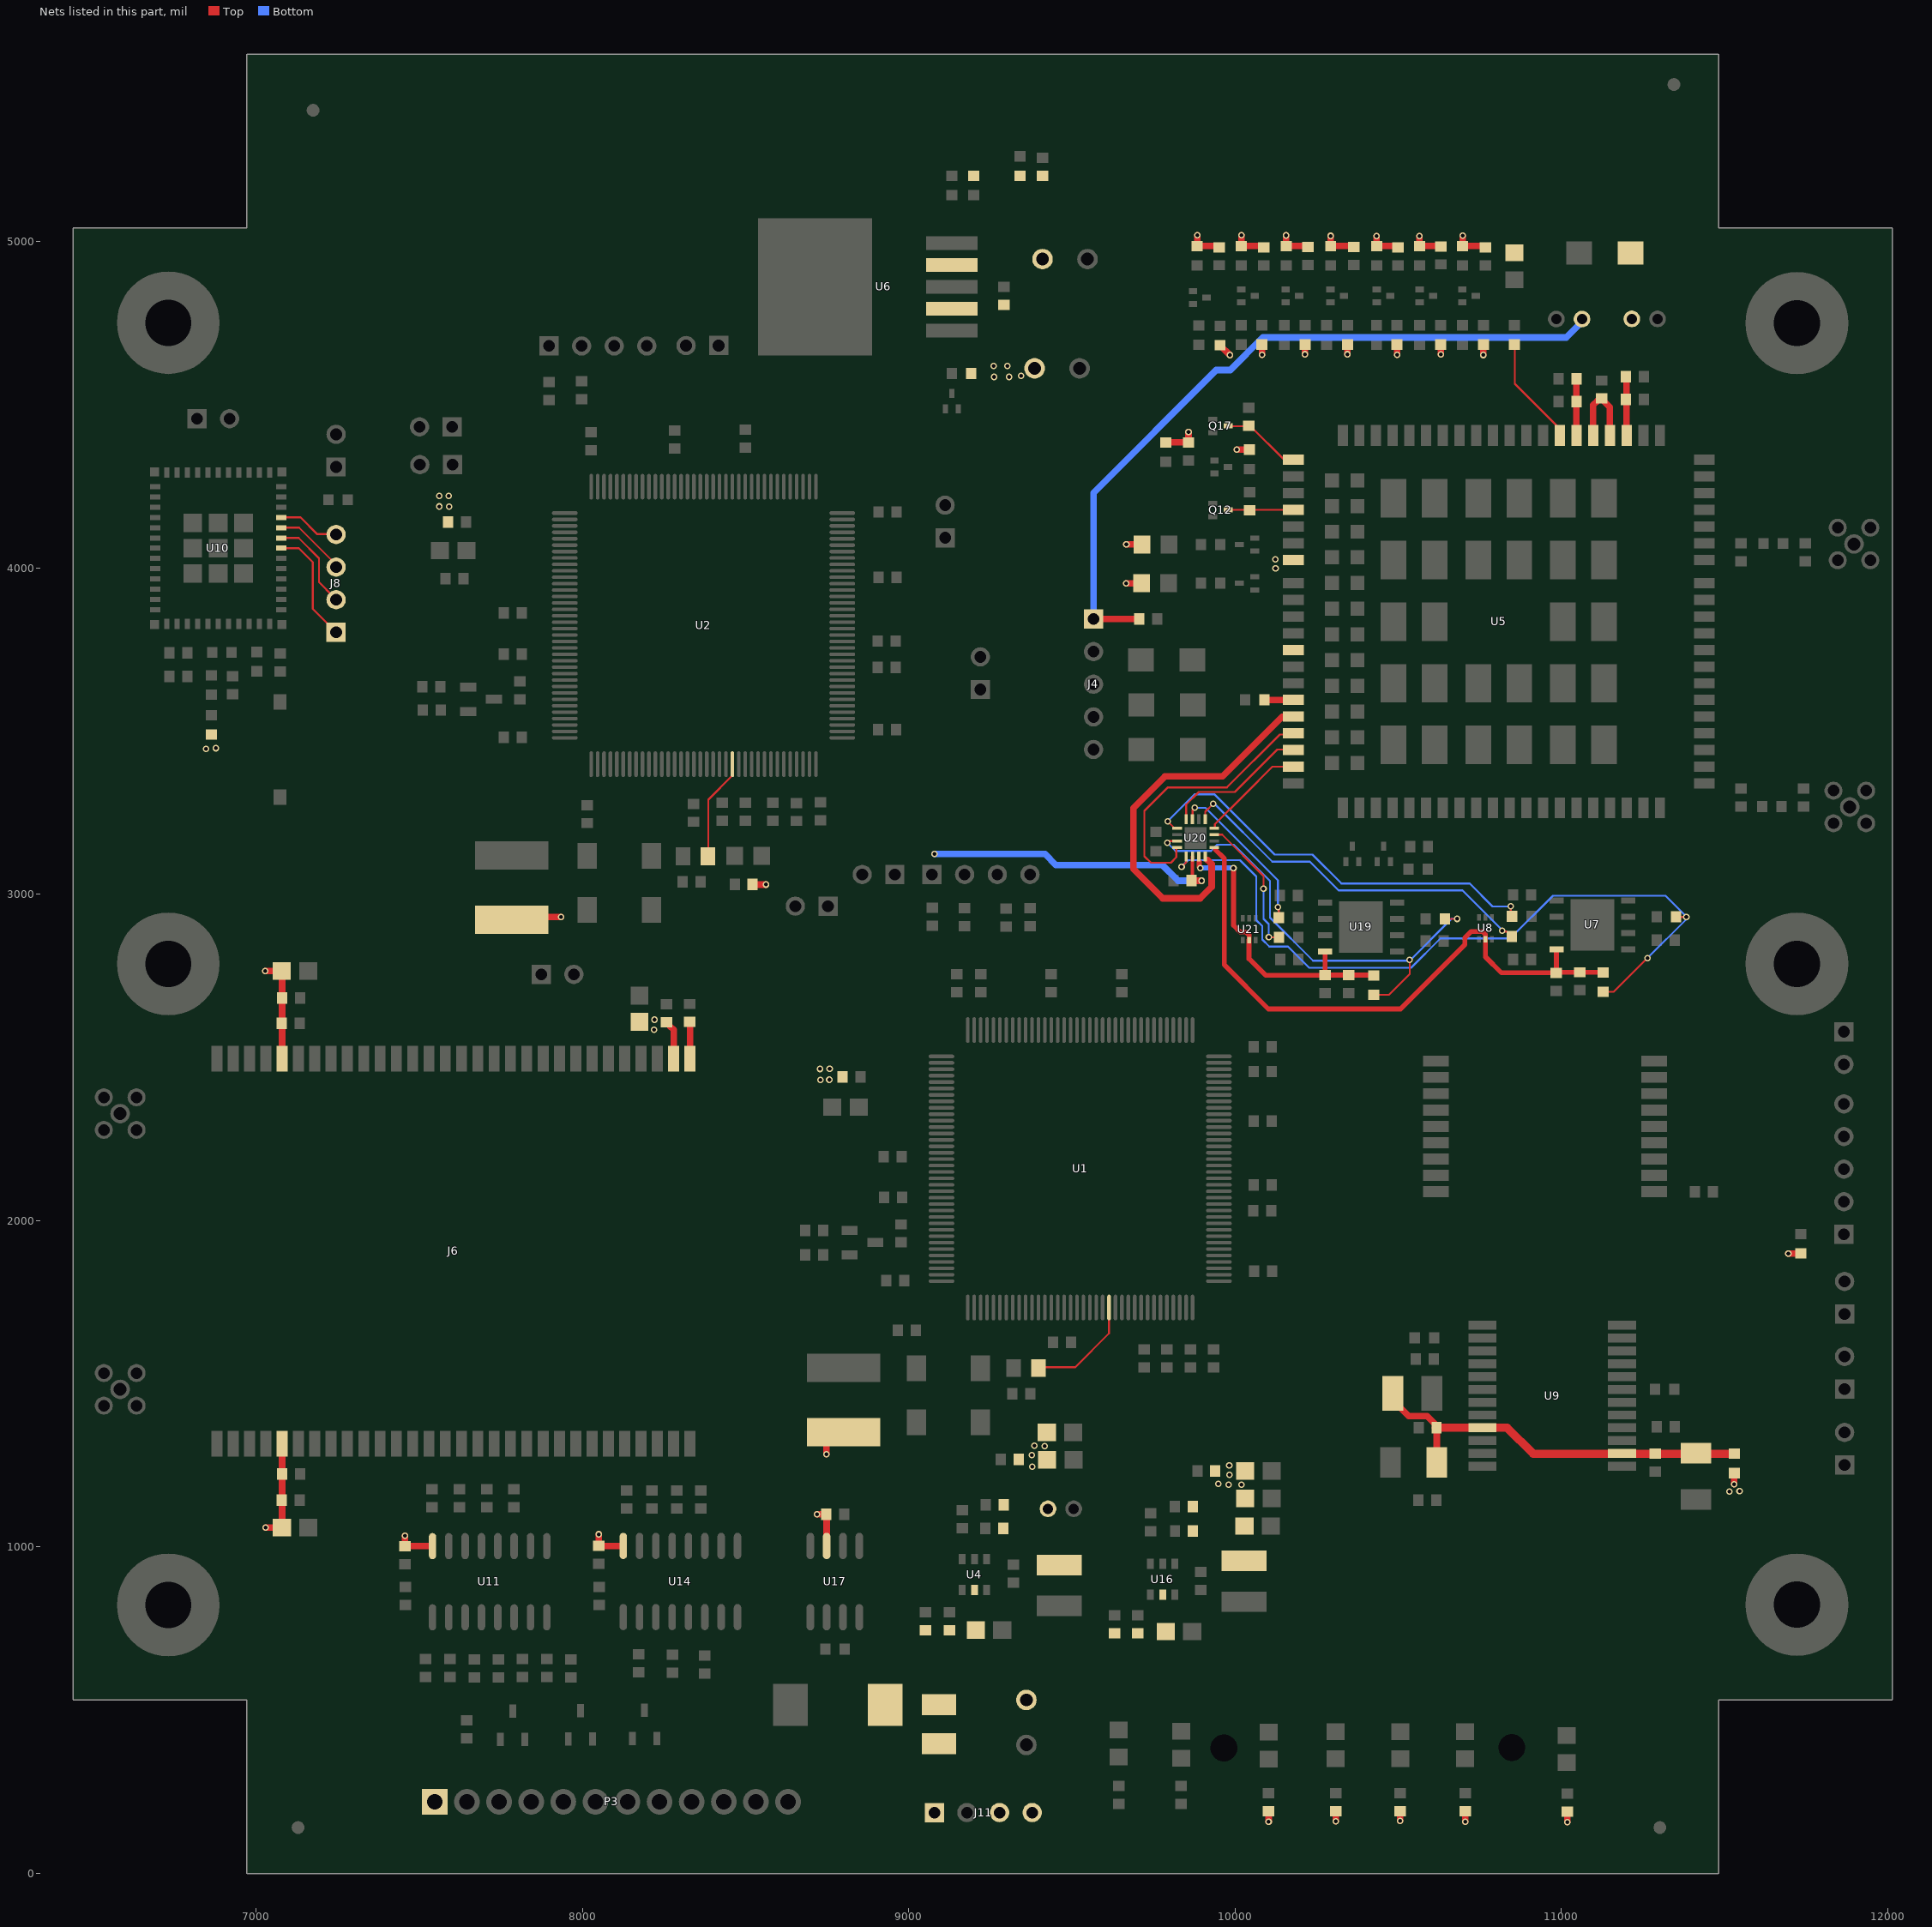
[diagram p0: the nets of this part, all layers, seen from the top]
# Altium PCB MISC86294.PcbDoc (part 7 of 8)
Units mil, origin at the board's own origin, x right, y up, seen from the top; angles counter-clockwise.
Board outline 5574.84 x 5574.84 mil, 4 copper layers (Top, GND02, PWR03, Bottom), stack 23.756 mil thick; 313 components, 311 nets, 1350 pads, 1701 vias.

## Via types
v1: diameter 20, hole 12, Top to Bottom, 1701 vias

## Nets (pads, with @x,y where several pads share a name; then routed paths per layer and width w, separated by ;. In a path a pad name is that pad's centre, name@x,y a point inside that pad or via, vN(x,y) a via of type N, cw(c..) or ccw(c..) an arc to the next point about the centre after c; other vN are vias at no path point) (continued)
SCC_VDD: C36.1 C37.1 C94.1 C95.1 L2.1 R22.2 U9.9 U9.14 | length 1194.8
  Top w20: L2.1@10503,1430 10532,1401 10588,1401 10617.42,1371.58 C94.1@10617.42,1365.98 ; C37.1@10618.01,1259 C94.1@10618.01,1361.01 ; R22.2@11529.87,1286.25 R22.2@11530.75,1286.25
  Top w25: C94.1@10615,1365 U9.9@10758.02,1364.99 10834,1365 10913.33,1285.67 R22.2@11529.87,1285.67
STATUS: R64.2 U5.61 | length 336.3
  Top w6: R64.2@10857,4686 10857,4565 10995,4427 U5.61@10995,4406.86
TCK: J8.3 U10.20 | length 216.3
  Top w6: U10.20@7075.91,4123.99 7131.01,4123.99 J8.3@7245,4010
TDI: J8.2 U10.19 | length 278.6
  Top w6: U10.19@7075.91,4092.5 7129.5,4092.5 7192,4030 7192,3957 J8.2@7237,3912
TDO: J8.4 U10.21 | length 176.4
  Top w6: U10.21@7075.91,4155.49 7135.51,4155.49 7187,4104 J8.4@7231,4104
TMS: J8.1 U10.18 | length 338.5
  Top w6: U10.18@7075.91,4061 7130,4061 7173,4018 7173,3875 J8.1@7230,3818
USIM_CLK: U5.16 U20.8 | length 436.1
  Top w6: U20.8@9850,3237 9850,3275 9889,3314 9999,3314 10129,3444 U5.16@10168,3444 ; U5.16@10168,3442.31 U5.16@10178.08,3442.31
USIM_DATA: U5.15 U20.12 | length 840.3
  Top w6: U20.12@9820,3143 9820,3114 9803,3097 9742,3097 9722,3117 9722,3256 9794,3328 9975,3328 10137,3490 U5.15@10184,3490
USIM_GND: U5.10
USIM_PRESENCE: R62.2 U5.13 | length 81.9
  Top w20: R62.2@10096.16,3595.85 U5.13@10178.08,3595.85
USIM_RST: U5.17 U20.4 | length 329.7
  Top w6: U20.4@9938,3204 9938,3215 10029,3306 ; 10025,3302 10029,3306 ; U5.17@10178.08,3391.12 10114.12,3391.12 10029,3306
USIM_VDD: U5.14 U20.16 | length 1171.7
  Top w20: 9916,3105 9928,3093 9928,3023 9893,2988 9778,2988 9688,3078 9688,3265 9785,3362 9962,3362 10144.67,3544.66 U5.14@10178.08,3544.66
USIMA_CLK: R67.1 U20.9 | length 1291.8
  Top w6: v1(9793,3224) 9814.43,3202.57 U20.9@9822.07,3202.57 ; v1@10845,2956 10845,2936.6 R67.1@10848.67,2932.92
  Bottom w6: v1(9793,3224) 9876,3307 9936,3307 10121,3122 10237,3122 10326,3033 10719,3033 10789,2963 v1@10842,2963 ; v1@10844,2965 10845,2965 v1(10845,2964) v1@10844,2965
USIMA_DATA: R69.1 R86.1 U20.13 | length 2337.2
  Top w6: v1(9836,3085) 9849.63,3098.63 U20.13@9849.63,3115.96 ; R86.1@11127.87,2701.36 11160.36,2701.36 v1(11264,2805) ; R69.1@11351.31,2931 v1(11383,2931)
  Bottom w6: v1(9836,3085) 9856,3105 10015,3105 10065,3055 10065,2921 10083,2903 10083,2862 10105,2840 10162,2840 10227,2775 10539,2775 10629,2865 10843,2865 10974,2996 11319,2996 v1@11384,2931 ; v1(11264,2805) 11382,2923 v1@11382,2932
USIMA_RST: R68.1 U20.5 | length 1127
  Top w6: U20.5@9908.67,3230.13 9908.67,3253.67 v1(9933,3278) ; v1@10820,2886 10832.12,2886 R68.1@10847.67,2870.45 R68.1@10846.55,2870.45
  Bottom w6: v1@9937,3277 10114,3100 10229,3100 10317,3012 10697,3012 v1@10813,2896
  other v1: 10818,2889
USIMA_VDD: C80.1 C83.1 R86.2 U7.8 U8.5 U20.1 | length 1846.7
  Top w15: 9939,3138 9967,3110 9967,2784 10102,2649 10507,2649 10704,2846 10704,2867 10723,2886 10754.77,2886 10754.89,2885.88 10756.89,2885.88 10757.89,2885.88 10758.81,2885.88 10764.69,2880 10765.19,2879.5 10767.28,2877.41 10767.28,2808.72 10816.42,2759.58 C83.1@10984.44,2759.58 ; C83.1@10984.79,2761.79 U7.8@10984.79,2831.5 ; C83.1@10989.25,2761.25 C80.1@11055.89,2761.25 R86.2@11124.25,2761.25
USIMB_CLK: R82.1 U20.7 | length 492.9
  Top w6: U20.7@9869.3,3230.13 9869.3,3259.3 v1(9876,3266) ; R82.1@10133.69,2929 v1@10133.69,2955.31
  Bottom w6: v1(9876,3266) v1@9879.5,3262.5 ; v1@9882,3265 9909,3265 10131,3043 v1(10131,2961)
USIMB_DATA: R87.2 R90.1 U20.11 | length 1414.2
  Top w6: v1(9792,3158) 9797.2,3163.2 U20.11@9822.07,3163.2 ; R87.2@10425.13,2692.33 10471.33,2692.33 10535,2756 v1(10535,2799) ; R90.1@10642.69,2925.1 v1@10678.1,2925.1
  Bottom w6: v1(9792,3158) 9817,3133 9926,3133 9945,3152 9996,3152 10107,3041 10107,2929 10239,2797 10535,2797 10664,2926 v1@10675,2926
  other v1: 10681,2925
USIMB_RST: R80.1 U20.3 | length 422.3
  Top w6: U20.3@9936.24,3182.95 9960.05,3182.95 10087,3056 v1(10087,3017) ; v1@10107.55,2868.45 R80.1@10134.67,2868.45
  Bottom w6: v1(10087,3017) 10087,2925 10103,2909 v1@10103,2875 ; v1@10100,2872 v1(10103,2869)
USIMB_VDD: C93.1 C128.1 R87.1 U19.8 U20.15 U21.5 | length 911.1
  Top w15: 9890,3100 9890,3084 v1(9893,3081) ; v1(9995,3081) 9995,2905 10015,2885 10033.77,2885 10043,2875.77 U21.5@10043,2859.53 ; U21.5@10042.72,2859.53 10042.72,2847.56 10042.72,2802.28 10048,2797 ; 10043.28,2802.72 10093.75,2752.25 C93.1@10275.89,2752.25 ; C93.1@10270.58,2752.58 C128.1@10347.55,2752.58 R87.1@10423.42,2752.58 ; C93.1@10275.59,2759.59 U19.8@10275.59,2825.03
  Bottom w15: v1(9893,3081) v1(9995,3081)
VBAT: C59.1 C60.1 C61.1 C62.1 C64.1 C65.1 C66.1 C67.1 C76.1 C77.1 D4.2 D8.1 J4.1 R60.2 R61.2 U5.57 U5.58 U5.59 U5.60 U6.4 | length 2777
  Top w20: J4.1@9590.35,3844.65 C62.1@9705.72,3844.65 ; U5.60@11046.18,4406.86 C66.1@11046.18,4565.82 ; U5.59@11097.37,4406.86 11097.37,4499.37 C61.1@11111,4513 ; C61.1@11129,4513 11148.55,4493.45 U5.58@11148.55,4406.86 ; C65.1@11199,4578 11199.73,4577.27 U5.57@11199.73,4406.86
  Bottom w20: J4.1@9565.93,3844.05 9565.93,4230.93 9942,4607 9985,4607 10085,4707 11015,4707 C59.1@11066,4758
VDD_3.3: C48.1 C49.1 C50.1 C51.1 C52.1 C99.2 C100.2 C101.2 C122.2 J6.31 J6.32 J11.4 L4.2 L200.2 L201.2 R6.1 R7.1 R9.1 R10.1 R19.1 R22.1 R25.1 R31.2 R32.2 R42.2 R44.2 R52.2 R55.2 R70.1 R84.1 R98.1 U20.14 | length 1684.4
  Top w10: C122.2@9869.31,3047.31 U20.14@9869.31,3115.95
  Top w20: L201.2@7870.56,2930.37 v1(7933.37,2930.37) ; C100.2@8268,2596 8279.01,2584.99 J6.32@8279.01,2496.94 ; J6.31@8329.01,2496.94 C99.2@8329.01,2602.01 ; R84.1@8521.25,3030.11 v1(8561.89,3030.11) ; v1(8746.83,1284.17) L200.2@8746.83,1348.63 ; C122.2@9866.86,3041.89 v1(9896.89,3041.89) ; v1(10082.1,4654.1) R44.2@10082.1,4685.14 ; v1(10102.81,158.19) R6.1@10102.81,190.46 ; v1(10308.07,158.93) R7.1@10308.07,190.46 ; v1(10496.3,4653.7) R42.2@10496.3,4685.14 ; v1(10505.52,160.48) R9.1@10505.52,190.46 ; v1(10630.09,4655.09) R52.2@10630.09,4685.14 ; v1(10705.6,157.4) R98.1@10705.6,190.46 ; v1(10760.89,4653.11) R55.2@10760.89,4685.14 ; v1(11017.89,156.11) R32.2@11017.89,189.14 ; v1(11529.87,1191.87) R22.1@11529.87,1226.36 ; v1(11695.64,1899.36) R25.1@11733.87,1899.36
  Bottom w20: v1(9079,3124) 9280.23,3124 9417,3124 9451,3090 9777,3090 9825.11,3041.89 v1(9896.89,3041.89)
  other v1: 11515,1170 11546,1171 9980,1191 10019,1191 9949,1193 9983,1221 9982,1250 8729,2431 8756,2432 8728,2465 8757.11,2465.89 8219,2585 8220,2616 6846,3446 6876,3448 7591,4188 7561,4189 7561,4221 7590,4221
VDD_5V: C39.1 C40.1 C41.1 C42.1 C43.1 C74.1 C75.1 C86.2 C87.1 C88.1 C89.2 C90.2 C91.2 C107.1 C111.1 C124.2 D9.1 D10.1 J6.5 J6.56 J11.3 L1.2 R27.2 R59.2 U6.2 U11.16 U14.16 U17.3 | length 1050.5
  Top w20: v1(7027.55,2765.45) C91.2@7077.99,2765.45 ; v1(7028.3,1059.3) C86.2@7078.15,1059.3 ; C86.2@7079.01,1067.01 J6.5@7079.01,1315.83 ; J6.56@7079.01,2496.94 C91.2@7079.01,2767.01 ; C107.1@7455.89,1002.25 v1(7455.89,1033.89) ; C107.1@7457.38,1002.38 U11.16@7540.02,1002.38 ; C111.1@8049.91,1003.05 v1(8049.91,1038.91) ; C111.1@8060.84,1003.16 8091,1003.16 U14.16@8124.68,1003.16 ; v1(8718.82,1100.18) C124.2@8747,1100.18 ; U17.3@8748,1003 C124.2@8748,1098 ; v1(9666.45,3953.45) D10.1@9713.1,3953.45 ; v1(9666.55,4072.45) D9.1@9714.1,4072.45
  other v1: 9378,1246 9377,1281 9416,1309 9385,1310 9261,4586 9307,4586 9344,4589 9260,4620 9302,4620
VDD_12V: C44.2 C45.2 C46.1 C53.2 C92.2 D1.2 R26.2 R29.1 R30.2 U4.5 U16.5
VDD_EXT: C54.1 C57.1 C58.1 C63.2 C68.2 C71.2 C72.2 C73.2 R34.2 R35.2 R37.1 R38.2 R39.1 R40.1 R45.1 R49.1 R54.1 R56.1 R57.1 R58.1 U5.7 | length 890.7
  Top w20: R58.1@9788.05,4385.07 9835,4385.07 C73.2@9857.07,4385.07 ; C73.2@9857.15,4384.93 v1(9857.15,4417.15) ; v1(9883.79,5020.79) R35.2@9883.79,4987.36 C57.1@9947.64,4987.36 ; R39.1@9953.8,4683.14 v1(9983.94,4653) ; v1(10004.77,4363.23) R57.1@10043.67,4363.23 ; v1(10018.97,5019.97) R49.1@10018.97,4987.36 C68.2@10083.64,4987.36 ; v1(10156.3,5019.7) R38.2@10156.3,4987.36 C58.1@10216.64,4987.36 ; v1(10214.45,4655.55) R40.1@10214.45,4685.14 ; v1(10292.73,5018.27) R34.2@10292.73,4987.36 C54.1@10353.64,4987.36 ; v1(10344.5,4655.5) R37.1@10344.5,4685.14 ; v1(10433.9,5018.1) R45.1@10433.9,4987.36 C63.2@10489.64,4987.36 ; v1(10565.08,5017.92) R54.1@10565.08,4987.36 C71.2@10622.64,4987.36 ; v1(10697.25,5019.25) R56.1@10697.25,4987.36 C72.2@10760.36,4987.36
  other v1: 10124,3999 10123,4027
VDD_IN: J11.1 P3.1 R29.2
W_DISABLE_MODULE: C78.1 Q12.3 U5.4 | length 197.6
  Top w6: Q12.3@9980.52,4178.52 U5.4@10178.08,4178.52
WAKEUP_IN_MODULE: C81.1 Q17.3 U5.1 | length 234.7
  Top w6: Q17.3@9986,4435 10047,4435 10149.93,4332.06 U5.1@10178.08,4332.06
XTAL1: R200.1 U1.23 | length 328.7
  Top w6: R200.1@9407,1551 9510,1551 9613.58,1654.58 U1.23@9613.58,1733.8
XTAL2: R201.1 U2.23 | length 301.8
  Top w6: R201.1@8385,3128 8385,3290.24 8459,3364.24 U2.23@8459,3371 ; U2.23@8459.19,3371 U2.23@8459.19,3399.13
pads on no net: J6.7 J6.8 J6.10 J6.11 J6.12 J6.13 J6.15 J6.16 J6.17 J6.19 J6.20 J6.21 J6.22 J6.26 J6.27 J6.28 J6.29 J6.30 J6.41 J6.42 J6.44 J6.45 J6.46 J6.48 J6.49 J6.50 J6.51 J6.53 J6.54 U1.7 U1.8 U1.9 U1.18 U1.19 U1.20 U1.21 U1.22 U1.24 U1.45 U1.46 U1.47 U1.49 U1.73 U1.74 U1.75 U1.76 U1.91 U1.92 U1.93 U1.98 U1.99 U1.100 U1.117 U1.124 U1.125 U1.126 U1.127 U1.132 U1.133 U1.134 U1.135 U1.136 U1.139 U1.140 U1.143 U2.7 U2.8 U2.9 U2.18 U2.19 U2.20 U2.21 U2.22 U2.24 U2.27 U2.28 U2.29 U2.40 U2.41 U2.42 U2.43 U2.44 U2.46 U2.47 U2.49 U2.73 U2.76 U2.91 U2.100 U2.103 U2.104 U2.106 U2.110 U2.117 U2.124 U2.125 U2.126 U2.127 U2.132 U2.133 U2.134 U2.135 U2.136 U2.139 U2.140 U3.4 U3.5 U3.10 U3.11 U3.12 U3.13 U3.14 U3.15 U3.16 U3.17 U3.18 U5.3 U5.18 U5.23 U5.24 U5.25 U5.26 U5.27 U5.28 U5.29 U5.30 U5.31 U5.32 U5.33 U5.34 U5.37 U5.38 U5.39 U5.40 U5.41 U5.42 U5.43 U5.44 U5.45 U5.47 U5.55 U5.69 U5.70 U5.71 U5.113 U5.114 U5.115 U5.116 U5.117 U5.118 U5.119 U5.120 U5.121 U5.122 U5.123 U5.124 U5.125 U5.126 U5.127 U5.128 U5.129 U5.130 U5.131 U5.132 U5.133 U5.134 U5.135 U5.136 U5.137 U5.138 U5.139 U5.140 U5.141 U5.142 U5.143 U5.144 U7.2 U7.4 U7.5 U8.6 U9.2 U9.11 U9.20 U9.21 U9.22 U9.23 U10.4 U10.6 U10.7 U10.9 U10.10 U10.12 U10.13 U10.14 U10.15 U10.16 U10.17 U10.24 U10.25 U10.28 U10.29 U10.32 U10.33 U10.34 U10.35 U14.7 U14.8 U14.9 U14.10 U17.5 U19.2 U19.4 U19.5 U21.6 Y1.1 Y2.1

## Polygon pours and split planes (outlines as drawn)
VDD_3.3 on Top "BottomLayer-No Net" (solid, remove dead copper, pour order 1027): 9853,1118 9853,1034 9857,1030 9880,1030 9905,1030 9910,1035 9910,1100 9910,1163 9915,1168 9921,1174 9949,1174 9955,1174 9960,1169 9970,1159 9970,1136 9970,1045 9955,1030 9950,1025 9950,970 9950,932 9959,923 9961,921 10011,921 10102,921 10109,928 10113,932 10113,945 10113,975 10085,1003 10059,1029 10059,1057 10059,1269 10054,1274 10048,1280 10036,1280 9934,1280 9928,1274 9922,1268 9922,1242 9922,1207 9905,1190 9853,1138 9853,1118
VDD_5V on Top "BottomLayer-No Net" (solid, remove dead copper, pour order 1025): 9271,1113 9271,1041 9274,1038 9277,1035 9297,1035 9309,1035 9315,1041 9317,1043 9317,1073 9317,1189 9317,1196 9326,1205 9331,1210 9343,1210 9364,1210 9367,1207 9383,1191 9383,1133 9383,922 9393,912 9397,908 9418,908 9530,908 9536,914 9544,922 9544,952 9544,986 9469,1061 9452,1078 9452,1261 9452,1376 9449,1379 9444,1384 9423,1384 9386,1384 9381,1379 9377,1375 9377,1360 9377,1324 9371,1318 9361,1308 9346,1308 9333,1308 9326,1301 9320,1295 9320,1277 9320,1243 9302,1225 9271,1194 9271,1113
NetC47_1 on Top "BottomLayer-No Net" (solid, remove dead copper, pour order 1024): 9804,858 9804,824 9811,817 9837,791 9942,791 10093,791 10100,798 10106,804 10106,818 10106,857 10099,864 10097,866 10080,866 9942,866 9925,883 9922,886 9901,886 9871,886 9863,878 9856,871 9833,871 9807,871 9805,869 9804,868 9804,858
NetC38_1 on Top "BottomLayer-No Net" (solid, remove dead copper, pour order 1023): 9227,867 9227,830 9234,823 9245,812 9263,812 9316,812 9337,791 9356,772 9415,772 9527,772 9536,781 9548,793 9548,817 9548,840 9534,854 9531,857 9496,857 9396,857 9347,906 9346,907 9325,907 9292,907 9288,903 9272,887 9247,887 9232,887 9227,882 9227,867
VDD_12V on Top "BottomLayer-No Net" (solid, remove dead copper, pour order 1022): 8862,565 8862,462 8877,447 8880,444 8921,444 8978,444 8998,464 9012,478 9065,478 9543,478 9572,507 9602,537 9774,537 9815,578 9815,784 9791,808 9791,841 9791,867 9788,870 9786,872 9782,872 9769,872 9767,870 9765,868 9765,843 9765,795 9745,775 9722,752 9682,752 9576,752 9543,719 9513,689 9366,689 9250,689 9240,699 9235,704 9235,743 9235,792 9222,805 9213,814 9213,856 9213,885 9212,886 9211,887 9205,887 9191,887 9189,885 9188,884 9188,879 9188,803 9174,789 9148,763 9114,763 9017,763 8930,676 8862,608 8862,565
VDD_IN on Top "BottomLayer-No Net" (solid, remove dead copper, pour order 1021): 8987,288 8987,166 9002,151 9008,145 9069,145 9100,145 9108,153 9118,163 9118,189 9118,246 9142,270 9162,290 9162,336 9162,421 9155,428 9148,435 9132,435 9046,435 9033,422 8987,376 8987,288
GND_IN on Top "BottomLayer-No Net" (solid, remove dead copper, pour order 1020): 7623,407 7623,275 7615,267 7605,257 7605,221 7605,197 7619,183 7626,176 7642,176 7667,176 7677,186 7684,193 7684,226 7684,421 7677,428 7675,430 7662,430 7628,430 7626,428 7623,425 7623,406
VDD_3.3 on Top "BottomLayer-No Net" (solid, remove dead copper, pour order 1019): 6826,3480 6826,3443 6833,3436 6838,3431 6854,3431 6892,3431 6895,3434 6900,3439 6900,3465 6900,3498 6896,3502 6890,3508 6874,3508 6834,3508 6828,3502 6826,3500 6826,3481
VDD_3.3 on Top "BottomLayer-No Net" (solid, remove dead copper, pour order 1018): 11497,1214 11497,1175 11497,1169 11502,1164 11508,1158 11527,1158 11556,1158 11559,1161 11566,1168 11566,1184 11566,1240 11563,1243 11551,1243 11509,1243 11503,1237 11497,1231 11497,1213
VDD_3.3 on Top "BottomLayer-No Net" (solid, remove dead copper, pour order 1026): 8146,2606 8146,2572 8153,2565 8159,2559 8182,2559 8237,2559 8258,2580 8259,2581 8279,2581 8345,2581 8352,2588 8354,2590 8354,2601 8354,2618 8350,2622 8345,2627 8320,2627 8231,2627 8218,2640 8209,2640 8152,2640 8148,2636 8146,2634 8146,2607
VDD_3.3 on Top "BottomLayer-No Net" (solid, remove dead copper, pour order 1028): 8795,2485 8728,2485 8719,2476 8714,2471 8714,2449 8714,2421 8720,2415 8725,2410 8749,2410 8804,2410 8811,2417 8813,2419 8813,2429 8813,2475 8808,2480 8803,2485 8795,2485
VDD_3.3 on Top "BottomLayer-No Net" (solid, remove dead copper, pour order 1029): 7575,4236 7553,4236 7549,4232 7531,4214 7531,4185 7531,4127 7534,4124 7539,4119 7557,4119 7598,4119 7600,4121 7604,4125 7604,4135 7604,4226 7599,4231 7594,4236 7575,4236
MCU1_VCC on Top "BottomLayer-No Net" (solid, remove dead copper, pour order 1030): 8890,2466 8865,2466 8843,2466 8837,2460 8835,2458 8835,2449 8835,2402 8822,2389 8816,2383 8816,2361 8816,2319 8819,2316 8824,2311 8835,2311 8923,2311 8931,2319 8936,2324 8936,2351 8936,2449 8927,2458 8919,2466 8890,2466
MCU2_VCC on Top "BottomLayer-No Net" (solid, remove dead copper, pour order 1031): 7675,4168 7636,4168 7629,4161 7627,4159 7627,4152 7627,4098 7616,4087 7616,4057 7616,3944 7623,3937 7630,3930 7653,3930 7699,3930 7703,3934 7711,3942 7711,3967 7711,4157 7705,4163 7700,4168 7676,4168
VDD_5V on Top "BottomLayer-No Net" (solid, remove dead copper, pour order 1032): 9174,4599 9174,4578 9176,4576 9184,4568 9218,4568 9396,4568 9403,4575 9421,4593 9421,4643 9421,4752 9357,4816 9356,4817 9198,4817 9055,4817 9053,4815 9052,4814 9052,4808 9052,4779 9055,4776 9056,4775 9066,4775 9232,4775 9238,4769 9242,4765 9242,4748 9242,4655 9231,4644 9208,4621 9190,4621 9181,4621 9177,4617 9174,4614 9174,4599
VDD_EXT on Top "BottomLayer-No Net" (solid, remove dead copper, pour order 1033): 10106,4022 10106,3989 10109.89,3985 10112.81,3982 10119.61,3982 10131.28,3982 10143.93,3995 10154.62,4006 10187.69,4006 10204.22,4006 10209.08,4011 10212,4014 10212,4024 10212,4038 10209.08,4041 10208.11,4042 10198.39,4042 10117.67,4042 10111.83,4036 10106,4030 10106,4022
VBAT on Top "BottomLayer-No Net" (solid, remove dead copper, pour order 1034): 9051,4940 9051,4911 9054,4908 9056,4906 9078,4906 9418,4906 9433,4921 9443,4931 9443,4978 9443,5024 9476,5057 9488,5069 10114,5069 10795,5069 10805,5059 10823,5041 10823,5005 10823,4947 10827,4943 10831,4939 10839,4939 10883,4939 10887,4943 10890,4946 10890,4963 10890,5039 10899,5048 10915,5064 10935,5064 11129,5064 11146,5047 11170,5023 11170,4929 11170,4906 11148,4884 11137,4873 11101,4873 11070,4873 11041,4844 11030,4833 11030,4576 11030,4479 11037,4472 11038,4471 11075,4471 11125,4471 11126,4472 11130,4476 11130,4486 11130,4529 11126,4533 11124,4535 11117,4535 11083,4535 11078,4540 11063,4555 11063,4565 11063,4614 11076,4627 11084,4635 11134,4635 11165,4635 11172,4628 11180,4620 11180,4594 11180,4548 11170,4538 11168,4536 11156,4536 11138,4536 11132,4530 11125,4523 11125,4506 11125,4471 11128,4471 11203,4471 11210,4478 11215,4483 11215,4503 11215,4627 11227,4639 11246,4658 11246,4746 11246,4821 11285,4860 11299,4874 11299,4970 11299,5158 11279,5178 11235,5222 9313,5222 9185,5222 9182,5219 9180,5217 9180,5212 9180,5189 9181,5188 9183,5186 9192,5186 9242,5186 9248,5180 9262,5166 9262,5134 9262,4983 9252,4973 9230,4951 9190,4951 9056,4951 9052,4947 9051,4946 9051,4941
GND on Top "BottomLayer-No Net" (solid, remove dead copper, pour order 1035): 6166,5202 6166,39 6407,-202 6487,-282 7221,-282 12093,-282 12302,-73 12382,7 12382,950 12382,5363 11996,5749 11907,5838 11118,5838 6391,5838 6238,5685 6166,5613 6166,5226
GND on Bottom "BottomLayer-No Net" (solid, remove dead copper, pour order 1036): 6041,5453 6041,164 6372,-167 6461,-256 7346,-256 12008,-256 12161,-103 12282,18 12282,984 12282,5429 11968,5743 11734,5977 10052,5977 6565,5977 6049,5461
GND on GND02 (split plane): 11462.17,5042.79 11462.55,5038.87 11463.7,5035.1 11465.55,5031.63 11468.05,5028.58 11471.1,5026.08 11474.57,5024.23 11478.34,5023.08 11482.26,5022.7 11993.66,5022.7 11993.66,551.05 11482.26,551.05 11478.34,550.66 11474.57,549.52 11471.1,547.66 11468.05,545.16 11465.55,542.12 11463.7,538.64 11462.55,534.87 11462.17,530.95 11462.17,19.55 6990.52,19.55 6990.52,530.95 6990.13,534.87 6988.99,538.64 6987.13,542.12 6984.63,545.16 6981.59,547.66 6978.11,549.52 6974.34,550.66 6970.42,551.05 6459.02,551.05 6459.02,3319 6667,3319 6667,4622 6459.02,4622 6459.02,5022.7 6970.42,5022.7 6974.34,5023.08 6978.11,5024.23 6981.59,5026.08 6984.63,5028.58 6987.13,5031.63 6988.99,5035.1 6990.13,5038.87 6990.52,5042.79 6990.52,5554.19 11462.17,5554.19
VDD_3.3 on PWR03 (split plane): 218 vertices, not listed, extent 6459.02,19.55 11993.66,5554.19
VDD_5V on PWR03 (split plane): 9723.91,4429.82 9723.91,3972 9724.26,3969.39 9725.26,3966.96 9726.87,3964.87 9728.57,3963.57 9729.87,3961.87 9768.87,3922.87 9770.96,3921.27 9772.68,3920.55 9773.39,3920.26 9776,3919.91 10104.82,3919.91 10641.91,3382.82 10641.91,1625.18 10443.87,1427.13 10442.26,1425.04 10441.9,1424.17 10299.82,1282.09 9978,1282.09 9975.39,1281.74 9973.67,1281.03 9972.96,1280.74 9970.87,1279.13 9914.87,1223.13 9913.26,1221.04 9912.26,1218.61 9911.91,1216 9911.91,869.18 9865.87,823.13 9585.87,543.13 9331.87,289.13 9330.26,287.04 9329.26,284.61 9328.91,282 9328.91,20.09 9147.09,20.09 9147.09,272 9146.74,274.61 9145.74,277.04 9144.13,279.13 9067.13,356.13 9065.04,357.73 9062.61,358.74 9060,359.09 8269.09,359.09 8269.09,670 8268.74,672.61 8267.74,675.04 8266.13,677.13 7949.13,994.13 7947.04,995.74 7945.53,996.36 7945.04,996.74 7942.61,997.74 7940,998.09 7068.18,998.09 6961.09,1105.18 6961.09,2748.82 7015.18,2802.91 7136.82,2802.91 7255.91,2683.82 7255.91,1821 7256.26,1818.39 7257.26,1815.96 7258.87,1813.87 7657.87,1414.87 7659.96,1413.26 7662.39,1412.26 7665,1411.91 8193.82,1411.91 8468.87,1136.87 8470.96,1135.26 8471.67,1134.97 8473.39,1134.26 8476,1133.91 9105,1133.91 9107.61,1134.26 9110.04,1135.26 9112.13,1136.87 9402.13,1426.87 9403.43,1428.57 9405.13,1429.87 9490.18,1514.91 9905,1514.91 9907.61,1515.26 9910.04,1516.26 9912.13,1517.87 10054.13,1659.87 10055.74,1661.96 10056.45,1663.68 10056.74,1664.39 10057.09,1667 10057.09,2517 10056.74,2519.61 10055.74,2522.04 10054.13,2524.13 9625.13,2953.13 9623.04,2954.73 9620.61,2955.74 9618,2956.09 9118.09,2956.09 9118.09,3173 9117.74,3175.61 9117.03,3177.33 9116.74,3178.04 9115.13,3180.13 8983.13,3312.13 8982.09,3312.93 8982.09,4204 8981.74,4206.61 8980.74,4209.04 8979.13,4211.13 8838.26,4352 9203.18,4716.91 9436.82,4716.91
GND on PWR03 (split plane): 6938.24,2750.49 6938.26,2750.39 6939.27,2747.96 6940.87,2745.87 6940.91,2745.83 6940.91,1101 6941.26,1098.39 6942.27,1095.96 6943.87,1093.87 7056.87,980.87 7058.96,979.26 7060.68,978.55 7061.39,978.26 7064,977.91 7935.82,977.91 8230.87,682.87 8232.96,681.27 8233.83,680.9 8248.91,665.82 8248.91,359.09 7524,359.09 7521.39,358.74 7519.67,358.03 7518.96,357.73 7516.87,356.13 7445.87,285.13 7444.26,283.04 7443.26,280.61 7442.91,278 7442.91,19.55 6990.52,19.55 6990.52,530.95 6990.13,534.87 6988.99,538.64 6987.13,542.12 6984.63,545.16 6981.59,547.66 6978.11,549.52 6974.34,550.66 6970.42,551.05 6459.02,551.05 6459.02,2915.91 6772.82,2915.91
MCU2_VCC on PWR03 (split plane): 8334.87,4343.87 8336.96,4342.27 8339.39,4341.26 8342,4340.91 8820.82,4340.91 8961.91,4199.82 8961.91,3309.18 8810.82,3158.09 8123.18,3158.09 7918.13,3363.13 7916.04,3364.73 7913.61,3365.74 7911,3366.09 7611.18,3366.09 7546.09,3431.18 7546.09,3619 7546.09,3879.82 7722.13,4055.87 7723.74,4057.96 7724.74,4060.39 7725.09,4063 7725.09,4331.82 7914.18,4520.91 8157.82,4520.91
MCU1_VCC on PWR03 (split plane): 10036.91,2512.82 10036.91,1671.18 9900.82,1535.09 9486,1535.09 9483.39,1534.74 9480.96,1533.74 9478.87,1532.13 9394,1447.26 9059.13,1782.13 9057.04,1783.74 9054.61,1784.74 9052,1785.09 8794.18,1785.09 8716.09,1863.18 8716.09,1904 8716.09,2219.82 9007.13,2510.87 9008.74,2512.96 9009.03,2513.67 9009.74,2515.39 9010.09,2518 9010.09,2831.82 9114.18,2935.91 9613.82,2935.91
VDD_EXT on PWR03 (split plane): 10730.91,5036.82 10730.91,4900.18 10687.82,4857.09 10481,4857.09 10478.39,4856.74 10477.68,4856.45 10475.96,4855.73 10473.87,4854.13 10389.87,4770.13 10388.26,4768.04 10387.26,4765.61 10386.91,4763 10386.91,4663.18 10352.82,4629.09 10215.18,4629.09 10185.09,4659.18 10185.09,4672 10184.74,4674.61 10183.74,4677.04 10182.13,4679.13 10148.13,4713.13 10146.04,4714.73 10143.61,4715.74 10141,4716.09 10075,4716.09 10072.39,4715.74 10070.67,4715.03 10069.96,4714.73 10067.87,4713.13 10026.87,4672.13 10025.26,4670.04 10024.26,4667.61 10023.91,4665 10023.91,4547 10024.26,4544.39 10025.26,4541.96 10026.87,4539.87 10162.91,4403.82 10162.91,3989.18 10113.82,3940.09 10111.49,3940.09 10111.11,3940.24 10108.5,3940.59 10105.89,3940.24 10105.51,3940.09 9780.18,3940.09 9746.91,3973.36 9746.74,3974.61 9745.74,3977.04 9744.13,3979.13 9744.09,3979.17 9744.09,4434 9743.74,4436.61 9743.03,4438.33 9742.74,4439.04 9741.13,4441.13 9475.26,4707 9821.18,5052.91 10714.82,5052.91
VDD_IN on PWR03 (split plane): 9126.91,267.82 9126.91,19.55 7463.09,19.55 7463.09,273.82 7528.18,338.91 9055.82,338.91

## Keep-outs
Keep-Out Layer:
  lines w3.94: 6972.4,5178.61 6972.4,5572.31 ; 11480.28,5178.61 11480.28,5572.31 ; 6972.4,5572.31 6972.4,5040.81 6440.91,5040.81 6440.91,532.93 6972.4,532.93 6972.4,1.44 11480.28,1.44 11480.28,532.93 12011.78,532.93 12011.78,5040.81 11480.28,5040.81 11480.28,5572.31 ; 6972.4,5572.31 11480.28,5572.31

## Other copper
Top:
  rectangle net VBAT: 11054,4471 11199,4536
  pour cut-out: 6667,3805 7103,3805 7103,4321 6667,4321
  pour cut-out: 10247,3369 10285,3331 11306,3331 11322,3347 11322,4343 11305,4360 10271,4360 10247,4336
GND02 (plane layer: these items are gaps in the copper):
  rectangle: 6446,3319 6667,4622
PWR03 (plane layer: these items are gaps in the copper):
  rectangle: 6446,3319 6667,4622
  lines w20: 6453,2926 6777,2926 6948,2755 6948,2753 ; 7453,16 7453,278 7524,349 9060,349 9137,272 9137,5 ; 7536,3596 7536,3884 7715,4063 7715,4336 7910,4531 8162,4531 8342,4351 8825,4351 8972,4204 8972,3305 8815,3148 8119,3148 7911,3356 7607,3356 7536,3427 7536,3619 ; 7941,987 7942,987 8259,670 8259,357 ; 8238,690 7940,988 7284,988 7064,988 6951,1101 6951,2753 7011,2813 7141,2813 7266,2688 7266,1821 7665,1422 8198,1422 8476,1144 ; 8737,1144 8476,1144 ; 8828,4356 9199,4727 9441,4727 9734,4434 9734,3972 ; 8975,3305 8976,3305 9108,3173 9108,2950 ; 9138,10 9339,10 9339,282 9922,865 9922,1216 9978,1272 10304,1272 10451,1419 ; 9395,1434 9105,1144 8476,1144 ; 9463,4709 9817,5063 10719,5063 10741,5041 10741,4896 10692,4847 10481,4847 10397,4763 10397,4659 10357,4619 10211,4619 10175,4655 10175,4672 10141,4706 10075,4706 10034,4665 10034,4547 10173,4408 10173,3985 10118,3930 9776,3930 9737,3969 9737,3972 ; 9593,536 9873,816 ; 10108.5,3930.5 10652,3387 10652,1621 10451,1420 ; 8706,1859 8706,1904 8706,2224 9000,2518 9000,2836 9110,2946 9618,2946 10047,2517 10047,1667 9905,1525 9486,1525 9398,1437 9390,1437 9052,1775 8790,1775 8706,1859
Multi-Layer:
  pour cut-out: 6667,4622 6667,3319 6431,3319 6431,4622